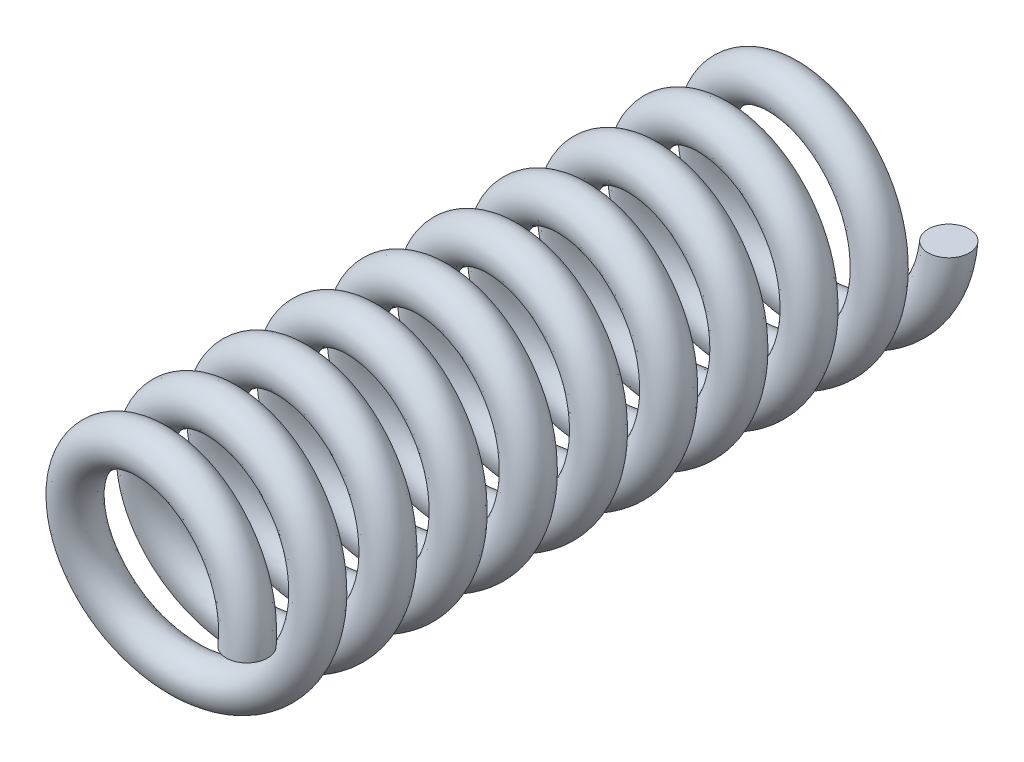
from build123d import *

# Parameters (mm, degrees)
SWEEP_1_PITCH  = 1.7
SWEEP_1_HEIGHT = 17
SWEEP_1_RADIUS = 2.5
SKETCH_2_R     = 0.5


with BuildPart() as part:
    # 扫描1: sweep along a helix
    with BuildLine() as sweep_1_path:
        Helix(SWEEP_1_PITCH, SWEEP_1_HEIGHT, SWEEP_1_RADIUS, center=(0, 0, 0), direction=(0, 0, 1), lefthand=True)
    # 草图2 → 扫描1 (sweep)
    with BuildSketch(Plane(origin=(0, 0, 0), x_dir=(1, 0, 0), z_dir=(0, 1, 0))):
        with Locations((2.5, 0)):
            Circle(SKETCH_2_R)
    sweep(path=sweep_1_path.line, is_frenet=True)


solid = part.part
